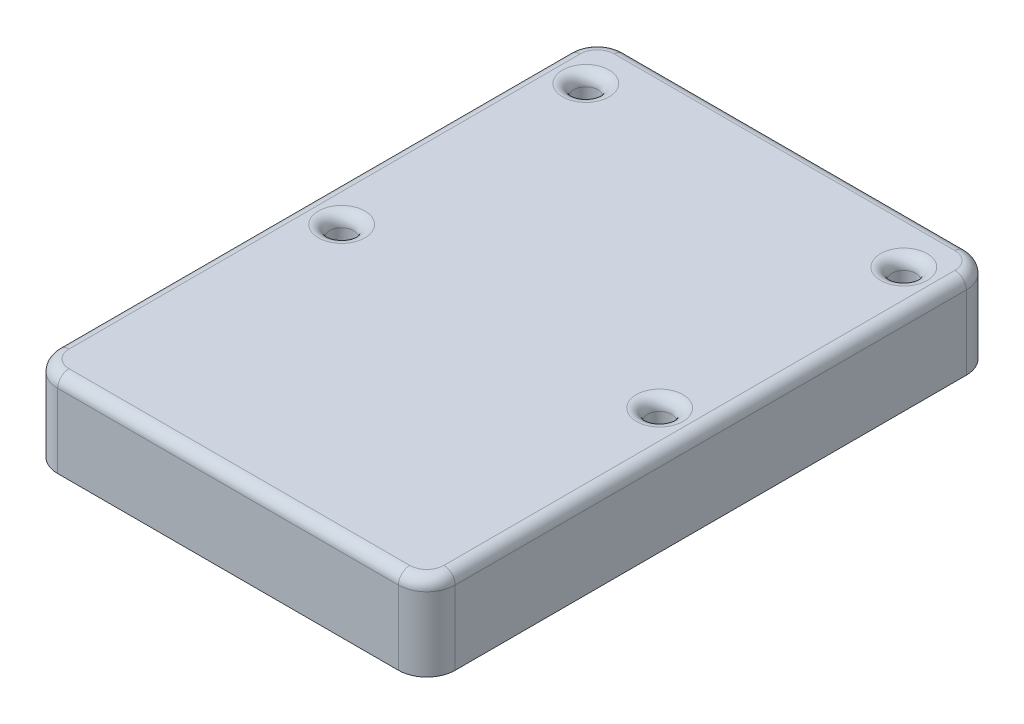
SolidWorks part; units mm, degrees
ref_plane "Front Plane" through (0, 0, 0) normal (0, 0, 1) x (1, 0, 0)
ref_plane "Top Plane" through (0, 0, 0) normal (0, 1, 0) x (1, 0, 0)
ref_plane "Right Plane" through (0, 0, 0) normal (1, 0, 0) x (0, 0, -1)
sketch "Sketch1" plane through (0, 0, 0) normal (0, 1, 0) x (1, 0, 0)
  line L1 (-30, -50) -> (30, -50)
  line L2 (-35, -45) -> (-35, 45)
  line L3 (-30, 50) -> (30, 50)
  line L4 (35, -45) -> (35, 45)
  line L5 (-35, -50) -> (35, 50) construction
  line L6 (-35, 50) -> (35, -50) construction
  arc A0 (-30, -50) -> (-35, -45) centre (-30, -45) cw
  arc A1 (30, -50) -> (35, -45) centre (30, -45) ccw
  arc A2 (30, 50) -> (35, 45) centre (30, 45) cw
  arc A3 (-35, 45) -> (-30, 50) centre (-30, 45) cw
  point P0 (0, 0)
  dimension "D3" = 5
  dimension "D1" = 70
  dimension "D2" = 100
extrude "Boss-Extrude1" add sketch "Sketch1" along normal blind 15
sketch "Sketch2" plane through (0, 0, 0) normal (0, -1, 0) x (1, 0, 0)
  line L1 (-27, -47) -> (27, -47)
  line L2 (-32, -42) -> (-32, 42)
  line L3 (-27, 47) -> (27, 47)
  line L4 (32, -42) -> (32, 42)
  line L5 (-32, -47) -> (32, 47) construction
  line L6 (-32, 47) -> (32, -47) construction
  arc A0 (-27, -47) -> (-32, -42) centre (-27, -42) cw
  arc A1 (27, -47) -> (32, -42) centre (27, -42) ccw
  arc A2 (27, 47) -> (32, 42) centre (27, 42) cw
  arc A3 (-32, 42) -> (-27, 47) centre (-27, 42) cw
  point P0 (0, 0)
  dimension "D3" = 5
  dimension "D1" = 64
  dimension "D2" = 94
extrude "Cut-Extrude1" cut sketch "Sketch2" against normal blind 12
sketch "Sketch3" plane through (0, 0, 0) normal (0, -1, 0) x (1, 0, 0)
  line L0 (-27, -48.55) -> (27, -48.55)
  line L1 (33.55, -42) -> (33.55, 42)
  line L2 (27, 48.55) -> (-27, 48.55)
  line L3 (-33.55, 42) -> (-33.55, -42)
  line L4 (-27, -47) -> (27, -47)
  line L5 (32, -42) -> (32, 42)
  line L6 (27, 47) -> (-27, 47)
  line L7 (-32, 42) -> (-32, -42)
  line L8 (-27, -47) -> (27, -47)
  line L9 (32, -42) -> (32, 42)
  line L10 (27, 47) -> (-27, 47)
  line L11 (-32, 42) -> (-32, -42)
  arc A0 (27, -48.55) -> (33.55, -42) centre (27, -42) ccw
  arc A1 (33.55, 42) -> (27, 48.55) centre (27, 42) ccw
  arc A2 (-27, 48.55) -> (-33.55, 42) centre (-27, 42) ccw
  arc A3 (-33.55, -42) -> (-27, -48.55) centre (-27, -42) ccw
  arc A4 (-32, -42) -> (-27, -47) centre (-27, -42) ccw
  arc A5 (27, -47) -> (32, -42) centre (27, -42) ccw
  arc A6 (32, 42) -> (27, 47) centre (27, 42) ccw
  arc A7 (-27, 47) -> (-32, 42) centre (-27, 42) ccw
  arc A8 (-32, -42) -> (-27, -47) centre (-27, -42) ccw
  arc A9 (27, -47) -> (32, -42) centre (27, -42) ccw
  arc A10 (32, 42) -> (27, 47) centre (27, 42) ccw
  arc A11 (-27, 47) -> (-32, 42) centre (-27, 42) ccw
  dimension "D1" = 0
  dimension "D2" = 1.55
extrude "Cut-Extrude2" cut sketch "Sketch3" against normal blind 1
sketch "Sketch4" plane through (0, 12, 0) normal (0, -1, 0) x (1, 0, 0)
  line L0 (32, -42) -> (32, 42) construction
  line L1 (-32, 42) -> (-32, -42) construction
  line L2 (-28, 6) -> (-32, 6)
  line L3 (-28, -2) -> (-32, -2)
  line L4 (28, 6) -> (32, 6)
  line L5 (28, -2) -> (32, -2)
  line L6 (-27, -47) -> (27, -47)
  line L7 (32, -42) -> (32, 42)
  line L8 (27, 47) -> (-27, 47)
  line L9 (-24, -41) -> (-24, -47)
  line L10 (-32, 42) -> (-32, -42)
  line L12 (32, -42) -> (32, -37)
  line L14 (-32, 6) -> (-32, -2)
  line L15 (30, -50) -> (-30, -50) construction
  line L16 (28, -37) -> (32, -37)
  line L18 (-28, -37) -> (-32, -37)
  line L19 (24, -41) -> (24, -47)
  line L20 (-32, -37) -> (-32, -42)
  line L21 (32, -2) -> (32, 6)
  line L22 (-27, -47) -> (27, -47) construction
  line L23 (-24, -47) -> (-27, -47)
  line L24 (24, -47) -> (27, -47)
  arc A0 (-24, -41) -> (-28, -37) centre (-28, -41) ccw
  arc A1 (28, -37) -> (24, -41) centre (28, -41) ccw
  arc A2 (28, 6) -> (28, -2) centre (28, 2) ccw
  arc A3 (-28, -2) -> (-28, 6) centre (-28, 2) ccw
  arc A4 (27, -47) -> (31, -45) centre (27, -42) ccw
  arc A8 (-32, -42) -> (-27, -47) centre (-27, -42) ccw
  arc A9 (27, -47) -> (32, -42) centre (27, -42) ccw
  arc A10 (32, 42) -> (27, 47) centre (27, 42) ccw
  arc A11 (-27, 47) -> (-32, 42) centre (-27, 42) ccw
  arc A12 (-32, -42) -> (-27, -47) centre (-27, -42) ccw
  arc A13 (31, -45) -> (32, -42) centre (27, -42) ccw
  dimension "D1" = 8
  dimension "D2" = 8
  dimension "D3" = 8
  dimension "D4" = 8
  dimension "D6" = 4
  dimension "D7" = 4
  dimension "D8" = 4
  dimension "D9" = 52
  dimension "D10" = 52
  dimension "D11" = 9
  dimension "D5" = 4
  dimension "D12" = 0
extrude "Boss-Extrude2" add sketch "Sketch4" along normal blind 11
sketch "Sketch5" plane through (0, 15, 0) normal (0, 1, 0) x (1, 0, 0)
  line L0 (35, -45) -> (35, 45) construction
  line L1 (30, 50) -> (-30, 50) construction
  line L2 (-35, 45) -> (-35, -45) construction
  line L3 (30, 50) -> (-30, 50) construction
  circle A0 centre (28, -2) radius 1.2
  circle A1 centre (28, 41) radius 1.2
  circle A2 centre (-28, 41) radius 1.2
  circle A3 centre (-28, -2) radius 1.2
  dimension "D1" = 2.4
  dimension "D2" = 2.4
  dimension "D3" = 2.4
  dimension "D4" = 2.4
  dimension "D5" = 7
  dimension "D6" = 7
  dimension "D7" = 9
  dimension "D8" = 7
  dimension "D9" = 7
  dimension "D10" = 52
  dimension "D11" = 52
  dimension "D12" = 9
extrude "Cut-Extrude3" cut sketch "Sketch5" against normal through all
sketch "Sketch6" plane through (0, 15, 0) normal (0, 1, 0) x (1, 0, 0)
  circle A0 centre (28, -2) radius 2.1
  circle A1 centre (-28, -2) radius 2.1
  circle A2 centre (-28, 41) radius 2.1
  circle A3 centre (28, 41) radius 2.1
  dimension "D1" = 4.2
  dimension "D2" = 4.2
  dimension "D3" = 4.2
  dimension "D4" = 4.2
extrude "Cut-Extrude4" cut sketch "Sketch6" against normal blind 12
fillet "Fillet1" radius 2 12 edges at (-35, 15, 0) (-33.5355, 15, -48.5355) (0, 15, -50) (33.5355, 15, -48.5355) (35, 15, 0) (33.5355, 15, 48.5355) (0, 15, 50) (-33.5355, 15, 48.5355) (28, 15, 4.1) (-28, 15, 4.1) (-28, 15, -38.9) (28, 15, -38.9)
scale "Scale1" scale about centroid uniform scaling yes scale factor 0.5
fillet "Fillet2" radius 1 8 edges at (-16, 8.5463, -19.2106) (16, 8.5463, -19.2106) (16, 8.5463, 2.2894) (16, 8.5463, -1.7106) (-16, 8.5463, -1.7106) (-16, 8.5463, 2.2894) (12, 8.5463, -24.2106) (-12, 8.5463, -24.2106)
